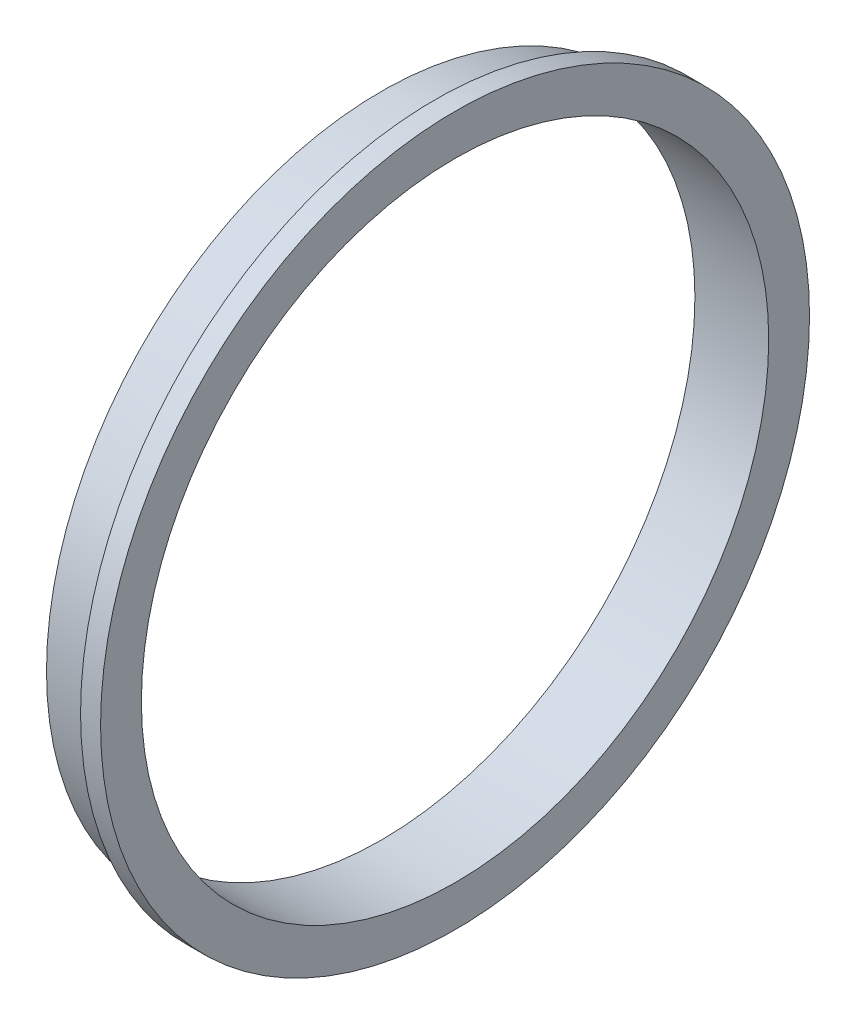
from build123d import *


with BuildPart() as part:
    # 草图1 → 旋转1 (revolve)
    with BuildSketch(Plane.XY, mode=Mode.PRIVATE) as revolve_1_sk:
        Polygon((0, 297.5), (70, 297.5), (70, 336.2), (51, 336.2), (51, 317.5), (0, 317.5), align=None)
    revolve(revolve_1_sk.sketch.rotate(Axis((-185.131578947, 0, 0), (1, 0, 0)), 90), axis=Axis((-185.131578947, 0, 0), (1, 0, 0)))


solid = part.part
